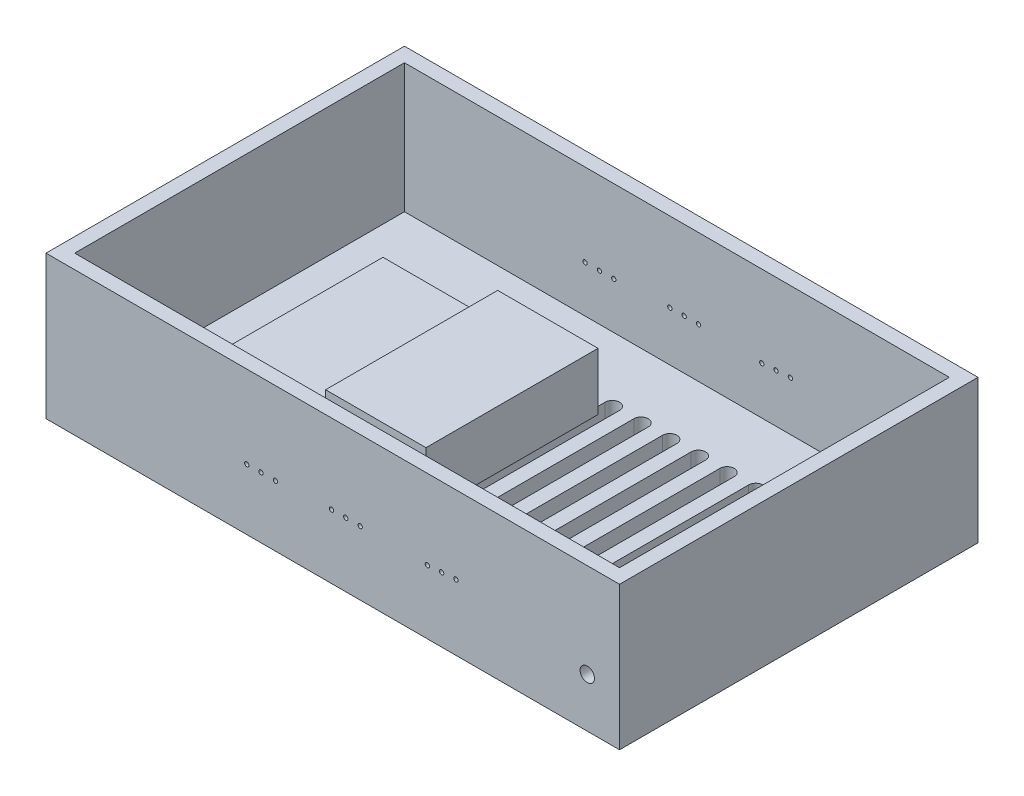
SolidWorks part; units mm, degrees
ref_plane "Front Plane" through (0, 0, 0) normal (0, 0, 1) x (1, 0, 0)
ref_plane "Top Plane" through (0, 0, 0) normal (0, 1, 0) x (1, 0, 0)
ref_plane "Right Plane" through (0, 0, 0) normal (1, 0, 0) x (0, 0, -1)
other "Configuration Table"
sketch "Sketch1" plane through (0, 0, 0) normal (0, 0, 1) x (1, 0, 0)
  line L1 (-200, 50) -> (200, 50)
  line L2 (-200, 50) -> (-200, -50)
  line L3 (-200, -50) -> (200, -50)
  line L4 (200, 50) -> (200, -50)
  line L5 (-200, 50) -> (200, -50) construction
  line L6 (-200, -50) -> (200, 50) construction
  point P0 (0, 0)
  dimension "D1" = 400
  dimension "D2" = 100
extrude "Boss-Extrude1" add sketch "Sketch1" along normal mid plane 250
shell "Shell1" thickness 10
sketch "Sketch2" plane through (0, 0, 125) normal (0, 0, 1) x (1, 0, 0)
  line L0 (-60, -7.5) -> (-50.0696, -7.4689) construction
  line L1 (-50.0696, -7.4689) -> (-40, -7.5) construction
  line L2 (-40, -7.5) -> (-0.8934, -5.3058) construction
  line L3 (-0.8934, -5.3058) -> (9.0324, -5.2727) construction
  line L4 (9.0324, -5.2727) -> (19.1066, -5.3058) construction
  line L5 (19.1066, -5.3058) -> (65.9645, -5.4787) construction
  line L6 (65.9645, -5.4787) -> (75.9416, -4.8022) construction
  line L7 (75.9416, -4.8022) -> (85.9187, -4.1257) construction
  circle A0 centre (-60, -7.5) radius 1.5
  circle A1 centre (-50.0696, -7.4689) radius 1.5
  circle A2 centre (-40, -7.5) radius 1.5
  circle A3 centre (-0.8934, -5.3058) radius 1.5
  circle A4 centre (9.0324, -5.2727) radius 1.5
  circle A5 centre (19.1066, -5.3058) radius 1.5
  circle A6 centre (65.9645, -5.4787) radius 1.5
  circle A7 centre (75.9416, -4.8022) radius 1.5
  circle A8 centre (85.9187, -4.1257) radius 1.5
  dimension "D1" = 3
  dimension "D2" = 60
  dimension "D3" = 7.5
extrude "Cut-Extrude1" cut sketch "Sketch2" against normal blind 20
sketch "Sketch6" plane through (0, -40, 0) normal (0, 1, 0) x (1, 0, 0)
  line L5 (-150, 60) -> (0, 60)
  line L6 (-150, 60) -> (-150, -60)
  line L7 (-150, -60) -> (0, -60)
  line L8 (0, 60) -> (0, -60)
  point P4 (0, 0)
  dimension "D1" = 150
  dimension "D2" = 120
extrude "Boss-Extrude2" add sketch "Sketch6" along normal blind 20
sketch "Sketch9" plane through (0, -40, 0) normal (0, 1, 0) x (1, 0, 0)
  line L0 (100, 70) -> (100, -70) construction
  line L1 (105, 70) -> (105, -70)
  line L2 (95, 70) -> (95, -70)
  line L3 (0, 0) -> (-90.1281, 0) construction
  line L4 (80, 70) -> (80, -70) construction
  line L5 (85, 70) -> (85, -70)
  line L6 (75, 70) -> (75, -70)
  line L7 (60, 70) -> (60, -70) construction
  line L8 (65, 70) -> (65, -70)
  line L9 (55, 70) -> (55, -70)
  line L10 (40, 70) -> (40, -70) construction
  line L11 (45, 70) -> (45, -70)
  line L12 (35, 70) -> (35, -70)
  line L13 (20, 70) -> (20, -70) construction
  line L14 (25, 70) -> (25, -70)
  line L15 (15, 70) -> (15, -70)
  line L16 (0, 70) -> (0, -70) construction
  line L17 (5, 70) -> (5, -70)
  line L18 (-5, 70) -> (-5, -70)
  line L19 (-20, 70) -> (-20, -70) construction
  line L20 (-15, 70) -> (-15, -70)
  line L21 (-25, 70) -> (-25, -70)
  line L22 (-40, 70) -> (-40, -70) construction
  line L23 (-35, 70) -> (-35, -70)
  line L24 (-45, 70) -> (-45, -70)
  line L25 (-60, 70) -> (-60, -70) construction
  line L26 (-55, 70) -> (-55, -70)
  line L27 (-65, 70) -> (-65, -70)
  line L28 (-80, 70) -> (-80, -70) construction
  line L29 (-75, 70) -> (-75, -70)
  line L30 (-85, 70) -> (-85, -70)
  line L31 (-100, 70) -> (-100, -70) construction
  line L32 (-95, 70) -> (-95, -70)
  line L33 (-105, 70) -> (-105, -70)
  line L34 (-120, 70) -> (-120, -70) construction
  line L35 (-115, 70) -> (-115, -70)
  line L36 (-125, 70) -> (-125, -70)
  line L37 (-140, 70) -> (-140, -70) construction
  line L38 (-135, 70) -> (-135, -70)
  line L39 (-145, 70) -> (-145, -70)
  line L40 (-160, 70) -> (-160, -70) construction
  line L41 (-155, 70) -> (-155, -70)
  line L42 (-165, 70) -> (-165, -70)
  arc A0 (105, 70) -> (95, 70) centre (100, 70) ccw
  arc A1 (95, -70) -> (105, -70) centre (100, -70) ccw
  arc A2 (85, 70) -> (75, 70) centre (80, 70) ccw
  arc A3 (75, -70) -> (85, -70) centre (80, -70) ccw
  arc A4 (65, 70) -> (55, 70) centre (60, 70) ccw
  arc A5 (55, -70) -> (65, -70) centre (60, -70) ccw
  arc A6 (45, 70) -> (35, 70) centre (40, 70) ccw
  arc A7 (35, -70) -> (45, -70) centre (40, -70) ccw
  arc A8 (25, 70) -> (15, 70) centre (20, 70) ccw
  arc A9 (15, -70) -> (25, -70) centre (20, -70) ccw
  arc A10 (5, 70) -> (-5, 70) centre (0, 70) ccw
  arc A11 (-5, -70) -> (5, -70) centre (0, -70) ccw
  arc A12 (-15, 70) -> (-25, 70) centre (-20, 70) ccw
  arc A13 (-25, -70) -> (-15, -70) centre (-20, -70) ccw
  arc A14 (-35, 70) -> (-45, 70) centre (-40, 70) ccw
  arc A15 (-45, -70) -> (-35, -70) centre (-40, -70) ccw
  arc A16 (-55, 70) -> (-65, 70) centre (-60, 70) ccw
  arc A17 (-65, -70) -> (-55, -70) centre (-60, -70) ccw
  arc A18 (-75, 70) -> (-85, 70) centre (-80, 70) ccw
  arc A19 (-85, -70) -> (-75, -70) centre (-80, -70) ccw
  arc A20 (-95, 70) -> (-105, 70) centre (-100, 70) ccw
  arc A21 (-105, -70) -> (-95, -70) centre (-100, -70) ccw
  arc A22 (-115, 70) -> (-125, 70) centre (-120, 70) ccw
  arc A23 (-125, -70) -> (-115, -70) centre (-120, -70) ccw
  arc A24 (-135, 70) -> (-145, 70) centre (-140, 70) ccw
  arc A25 (-145, -70) -> (-135, -70) centre (-140, -70) ccw
  arc A26 (-155, 70) -> (-165, 70) centre (-160, 70) ccw
  arc A27 (-165, -70) -> (-155, -70) centre (-160, -70) ccw
  point P2 (100, 0)
  point P14 (80, 0)
  point P21 (60, 0)
  point P28 (40, 0)
  point P35 (20, 0)
  point P42 (0, 0)
  point P49 (-20, 0)
  point P56 (-40, 0)
  point P63 (-60, 0)
  point P70 (-80, 0)
  point P77 (-100, 0)
  point P84 (-120, 0)
  point P91 (-140, 0)
  point P98 (-160, 0)
  dimension "D3" = 5
  dimension "D1" = 100
  dimension "D2" = 140
  dimension "D5" = 20
  dimension "D4" = 14
extrude "Cut-Extrude4" cut sketch "Sketch9" against normal blind 40
sketch "Sketch10" plane through (0, -20, 0) normal (0, 1, 0) x (1, 0, 0)
  line L0 (0, 60) -> (-150, 60) construction
  line L1 (0, -60) -> (-70, -60)
  line L2 (0, -60) -> (0, 60)
  line L3 (0, 60) -> (-70, 60)
  line L4 (-70, -60) -> (-70, 60)
  dimension "D1" = 70
extrude "Boss-Extrude4" add sketch "Sketch10" along normal blind 20
sketch "Sketch11" plane through (0, 0, 125) normal (0, 0, 1) x (1, 0, 0)
  line L0 (200, -50) -> (200, 50) construction
  line L1 (-200, -50) -> (200, -50) construction
  circle A0 centre (177.51, -15.63) radius 5
  dimension "D3" = 10
  dimension "D1" = 22.49
  dimension "D2" = 34.37
extrude "Cut-Extrude5" cut sketch "Sketch11" against normal blind 20 contours A0
sketch "Sketch12" plane through (0, 0, -125) normal (0, 0, -1) x (-1, 0, 0)
  line L0 (-200, -50) -> (-200, 50) construction
  line L1 (200, -50) -> (-200, -50) construction
  circle A0 centre (-173.59, -15.71) radius 5
  dimension "D3" = 10
  dimension "D1" = 26.41
  dimension "D2" = 34.29
extrude "Cut-Extrude6" cut sketch "Sketch12" against normal blind 20 contours A0
sketch "Sketch13" plane through (0, 0, -125) normal (0, 0, -1) x (-1, 0, 0)
  line L0 (-79.16, -5.57) -> (-69.1829, -6.2465) construction
  line L1 (-69.1829, -6.2465) -> (-59.2058, -6.9231) construction
  line L2 (-59.2058, -6.9231) -> (-15.0866, -5.3747) construction
  line L3 (-15.0866, -5.3747) -> (-5.0866, -5.3747) construction
  line L4 (-5.0866, -5.3747) -> (4.9134, -5.3747) construction
  line L5 (4.9134, -5.3747) -> (44.02, -7.5689) construction
  line L6 (44.02, -7.5689) -> (54.02, -7.5689) construction
  line L7 (54.02, -7.5689) -> (64.02, -7.5689) construction
  line L8 (200, -50) -> (-200, -50) construction
  circle A0 centre (-79.16, -5.57) radius 1.5
  circle A1 centre (-59.2058, -6.9231) radius 1.5
  circle A2 centre (-69.1829, -6.2465) radius 1.5
  circle A3 centre (64.02, -7.5689) radius 1.5
  circle A4 centre (54.02, -7.5689) radius 1.5
  circle A5 centre (44.02, -7.5689) radius 1.5
  circle A6 centre (4.9134, -5.3747) radius 1.5
  circle A7 centre (-5.0866, -5.3747) radius 1.5
  circle A8 centre (-15.0866, -5.3747) radius 1.5
  circle A9 centre (-173.59, -15.71) radius 5 construction
  circle A10 centre (-173.59, -15.71) radius 5 construction
  dimension "D3" = 3
  dimension "D1" = 94.43
  dimension "D2" = 44.43
extrude "Cut-Extrude7" cut sketch "Sketch13" against normal blind 20
